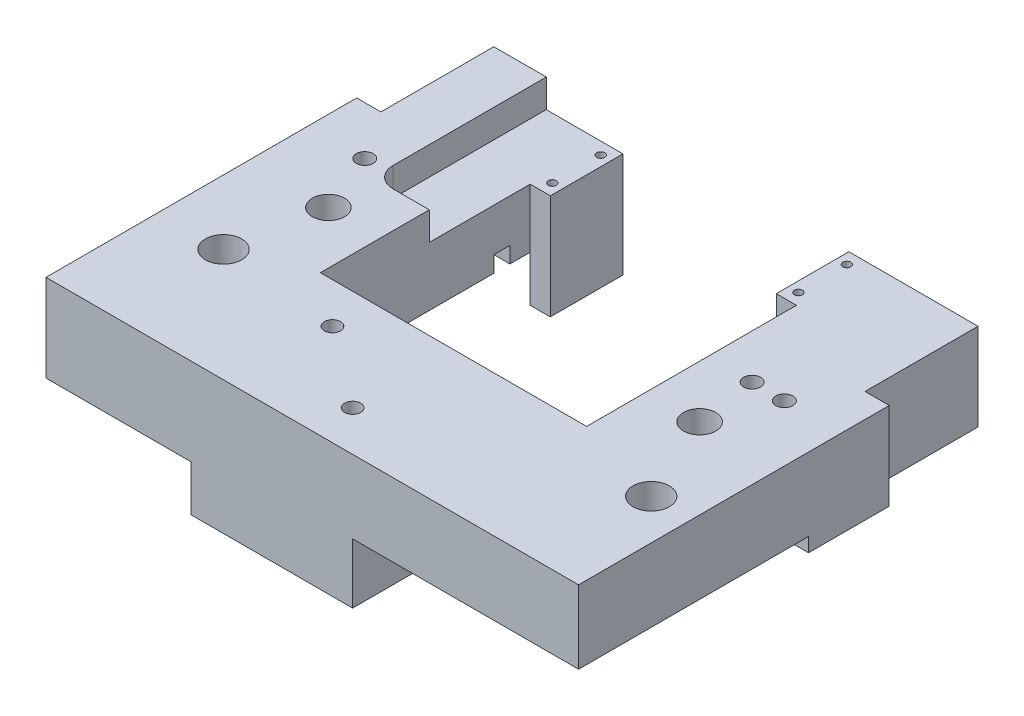
from build123d import *

# Parameters (mm, degrees)
SKETCH_1_W           = 132
SKETCH_1_H           = 33
EXTRUDE_1_DEPTH      = 105
CUT_EXTRUDE_1_REACH  = 135.792
CUT_EXTRUDE_2_DEPTH  = 11.37
CUT_EXTRUDE_3_REACH  = 135.792
SKETCH_4_W           = 6
SKETCH_4_H           = 28
SKETCH_5_W           = 57
SKETCH_5_H           = 3.5
CUT_EXTRUDE_5_DEPTH  = 56
SKETCH_7_W           = 4
SKETCH_7_H           = 4
CUT_EXTRUDE_6_DEPTH  = 166.956505693
CUT_EXTRUDE_7_DEPTH  = 7
SKETCH_9_R           = 2
SKETCH_9_R_2         = 4.5
SKETCH_9_R_3         = 4
SKETCH_9_R_4         = 2.1
SKETCH_9_R_5         = 1
CUT_EXTRUDE_8_DEPTH  = 134.79203893
SKETCH_10_R          = 7.5
CUT_EXTRUDE_9_DEPTH  = 13
SKETCH_11_R          = 2.5
CUT_EXTRUDE_10_DEPTH = 27
SKETCH_12_R          = 1.25
CUT_EXTRUDE_11_DEPTH = 8.5
SKETCH_13_R          = 1.65
CUT_EXTRUDE_12_DEPTH = 11.5
SKETCH_16_R          = 1.25
CUT_EXTRUDE_13_DEPTH = 8.5


with BuildPart() as part:
    # 草图1 → 凸台-拉伸1 (new body)
    with BuildSketch(Plane.XY):
        with Locations((-10.06779661, -8.809322034)):
            Rectangle(SKETCH_1_W, SKETCH_1_H)
    extrude(amount=EXTRUDE_1_DEPTH)

    # 草图2 → 切除-拉伸1 (cut, up to next)
    with BuildSketch(Plane(origin=(0, 7.690677966, 0), x_dir=(1, 0, 0), z_dir=(0, 1, 0)), mode=Mode.PRIVATE) as cut_extrude_1_sk1:
        Polygon((-43.06779661, -70), (22.93220339, -70), (22.93220339, -18), (17.93220339, -18), (17.93220339, 0), (-38.06779661, 0), (-38.06779661, -18), (-43.06779661, -18), align=None)
    cut_extrude_1_tool1 = extrude(cut_extrude_1_sk1.sketch, amount=-CUT_EXTRUDE_1_REACH, mode=Mode.PRIVATE) & part.part
    add(cut_extrude_1_tool1.solids().sort_by_distance((-10.067797, 7.690678, 36.054054))[0], mode=Mode.SUBTRACT)

    # 草图3 → 切除-拉伸2 (cut)
    with BuildSketch(Plane.XZ.offset(25.309322034)):
        Polygon((-0.06779661, 70), (-0.06779661, 105), (55.93220339, 105), (55.93220339, 28), (49.93220339, 28), (49.93220339, 0), (22.93220339, 0), (22.93220339, 70), align=None)
        Polygon((-40.06779661, 105), (-40.06779661, 70), (-43.06779661, 70), (-43.06779661, 0), (-70.06779661, 0), (-70.06779661, 28), (-76.06779661, 28), (-76.06779661, 105), align=None)
    extrude(amount=-CUT_EXTRUDE_2_DEPTH, mode=Mode.SUBTRACT)

    # 草图4 → 切除-拉伸3 (cut, up to next)
    with BuildSketch(Plane.XZ.offset(25.309322034), mode=Mode.PRIVATE) as cut_extrude_3_sk1:
        with Locations((-73.06779661, 14)):
            Rectangle(SKETCH_4_W, SKETCH_4_H)
    cut_extrude_3_tool1 = extrude(cut_extrude_3_sk1.sketch, amount=-CUT_EXTRUDE_3_REACH, mode=Mode.PRIVATE) & part.part
    # 草图4 → 切除-拉伸3 (cut, up to next)
    with BuildSketch(Plane.XZ.offset(25.309322034), mode=Mode.PRIVATE) as cut_extrude_3_sk2:
        with Locations((52.93220339, 14)):
            Rectangle(SKETCH_4_W, SKETCH_4_H)
    cut_extrude_3_tool2 = extrude(cut_extrude_3_sk2.sketch, amount=-CUT_EXTRUDE_3_REACH, mode=Mode.PRIVATE) & part.part
    add(cut_extrude_3_tool1.solids().sort_by_distance((-73.067797, -25.309322, 14))[0], mode=Mode.SUBTRACT)
    add(cut_extrude_3_tool2.solids().sort_by_distance((52.932203, -25.309322, 14))[0], mode=Mode.SUBTRACT)

    # 草图5 → 切除-拉伸5 (cut)
    with BuildSketch(Plane(origin=(55.93220339, 0, 0), x_dir=(0, 0, -1), z_dir=(1, 0, 0))):
        with Locations((-76.5, -12.189322034)):
            Rectangle(SKETCH_5_W, SKETCH_5_H)
    extrude(amount=-CUT_EXTRUDE_5_DEPTH, mode=Mode.SUBTRACT)

    # 草图7 → 切除-拉伸6 (cut, through all)
    with BuildSketch(Plane(origin=(49.93220339, 0, 0), x_dir=(0, 0, -1), z_dir=(1, 0, 0))):
        with Locations((-25, -11.939322034)):
            Rectangle(SKETCH_7_W, SKETCH_7_H)
    extrude(amount=-CUT_EXTRUDE_6_DEPTH, mode=Mode.SUBTRACT)

    # 草图8 → 切除-拉伸7 (cut)
    with BuildSketch(Plane(origin=(0, 7.690677966, 0), x_dir=(1, 0, 0), z_dir=(0, 1, 0))):
        with BuildLine():
            Line((-38.06779661, -18), (-43.06779661, -18))
            Line((-43.06779661, -18), (-43.06779661, -43))
            Line((-43.06779661, -43), (-52.06779661, -43))
            ThreePointArc((-52.06779661, -43), (-55.603330516, -41.535533906), (-57.06779661, -38))
            Line((-57.06779661, -38), (-57.06779661, 0))
            Line((-57.06779661, 0), (-38.06779661, 0))
            Line((-38.06779661, 0), (-38.06779661, -18))
        make_face()
    extrude(amount=-CUT_EXTRUDE_7_DEPTH, mode=Mode.SUBTRACT)

    # 草图9 → 切除-拉伸8 (cut, through all)
    with BuildSketch(Plane.XZ.offset(25.309322034)):
        with Locations(Location((-10.06779661, 95, 0), (0, 0, 270))):
            Circle(SKETCH_9_R)
        with Locations(Location((-30.06779661, 80, 0), (0, 0, 270))):
            Circle(SKETCH_9_R)
        with Locations(Location((-60.06779661, 77, 0), (0, 0, 270))):
            Circle(SKETCH_9_R_2)
        with Locations(Location((-56.06779661, 55, 0), (0, 0, 270))):
            Circle(SKETCH_9_R_3)
        with Locations(Location((-54.06779661, 40, 0), (0, 0, 90))):
            Circle(SKETCH_9_R_4)
        with Locations(Location((-62.06779661, 40, 0), (0, 0, 270))):
            Circle(SKETCH_9_R_4)
        with Locations(Location((-40.56779661, 15, 0), (0, 0, 270))):
            Circle(SKETCH_9_R_5)
        with Locations(Location((-40.56779661, 3, 0), (0, 0, 270))):
            Circle(SKETCH_9_R_5)
        with Locations(Location((45.93220339, 77, 0), (0, 0, 270))):
            Circle(SKETCH_9_R_2)
        with Locations(Location((35.93220339, 55, 0), (0, 0, 270))):
            Circle(SKETCH_9_R_3)
        with Locations(Location((20.43220339, 15, 0), (0, 0, 270))):
            Circle(SKETCH_9_R_5)
        with Locations(Location((20.43220339, 3, 0), (0, 0, 270))):
            Circle(SKETCH_9_R_5)
        with Locations(Location((41.93220339, 40, 0), (0, 0, 270))):
            Circle(SKETCH_9_R_4)
        with Locations(Location((33.93220339, 40, 0), (0, 0, 270))):
            Circle(SKETCH_9_R_4)
    extrude(amount=-CUT_EXTRUDE_8_DEPTH, mode=Mode.SUBTRACT)

    # 草图10 → 切除-拉伸9 (cut)
    with BuildSketch(Plane.XZ.offset(13.939322034)):
        with Locations(Location((-60.06779661, 77, 0), (0, 0, 270))):
            Circle(SKETCH_10_R)
        with Locations(Location((45.93220339, 77, 0), (0, 0, 270))):
            Circle(SKETCH_10_R)
    extrude(amount=-CUT_EXTRUDE_9_DEPTH, mode=Mode.SUBTRACT)

    # 草图11 → 切除-拉伸10 (cut)
    with BuildSketch(Plane.XZ.offset(25.309322034)):
        with Locations(Location((-30.06779661, 95, 0), (0, 0, 270))):
            Circle(SKETCH_11_R)
        with Locations(Location((-10.06779661, 80, 0), (0, 0, 270))):
            Circle(SKETCH_11_R)
    extrude(amount=-CUT_EXTRUDE_10_DEPTH, mode=Mode.SUBTRACT)

    # 草图12 → 切除-拉伸11 (cut)
    with BuildSketch(Plane.XZ.offset(10.439322034)):
        with Locations((34.48220339, 97.6)):
            Circle(SKETCH_12_R)
        with Locations((34.48220339, 71.6)):
            Circle(SKETCH_12_R)
    extrude(amount=-CUT_EXTRUDE_11_DEPTH, mode=Mode.SUBTRACT)

    # 草图13 → 切除-拉伸12 (cut)
    with BuildSketch(Plane.XZ.offset(13.939322034)):
        with Locations(Location((-68.06779661, 97, 0), (0, 0, 270))):
            Circle(SKETCH_13_R)
    extrude(amount=-CUT_EXTRUDE_12_DEPTH, mode=Mode.SUBTRACT)

    # 草图16 → 切除-拉伸13 (cut)
    with BuildSketch(Plane.XZ.offset(25.309322034)):
        with Locations(Location((-40.56779661, 9, 0), (0, 0, 270))):
            Circle(SKETCH_16_R)
        with Locations(Location((20.43220339, 9, 0), (0, 0, 270))):
            Circle(SKETCH_16_R)
    extrude(amount=-CUT_EXTRUDE_13_DEPTH, mode=Mode.SUBTRACT)


solid = part.part
